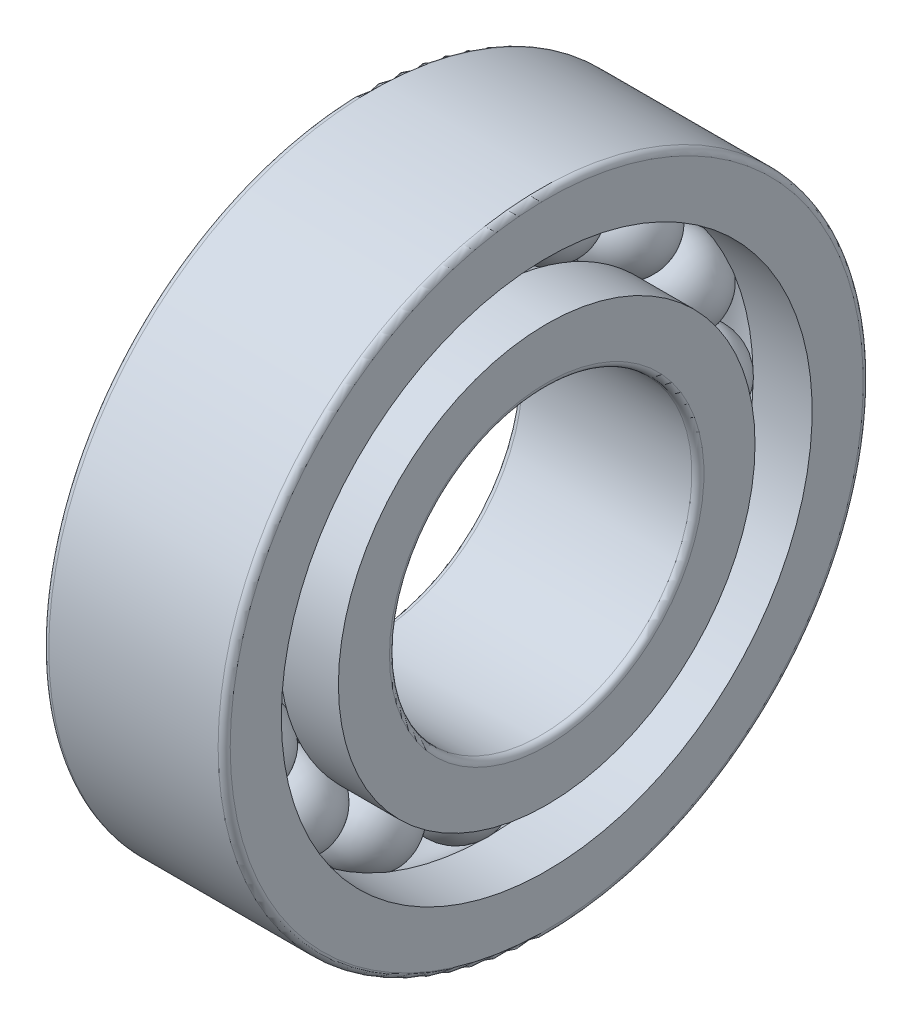
SolidWorks part; units mm, degrees
ref_plane "Front" through (0, 0, 0) normal (0, 0, 1) x (1, 0, 0)
ref_plane "Top" through (0, 0, 0) normal (0, 1, 0) x (1, 0, 0)
ref_plane "Right" through (0, 0, 0) normal (1, 0, 0) x (0, 0, -1)
sketch "Sketch1" plane through (0, 0, 0) normal (0, 0, 1) x (1, 0, 0)
  line L0 (-9.6833, 0) -> (9.8371, 0) construction
  line L1 (-2.125, 11.75) -> (2.125, 11.75)
  line L2 (-4.5966, 11.75) -> (4.6657, 11.75) construction
  arc A0 (2.125, 11.75) -> (-2.125, 11.75) centre (0, 11.75) ccw
revolve "Revolve1" add sketch "Sketch1" angle 360 about L2
sketch "Sketch2" plane through (0, 0, 0) normal (0, 0, 1) x (1, 0, 0)
  line L0 (-4.5, 10.3333) -> (-4.5, 7.5)
  line L1 (-4.5, 7.5) -> (4.5, 7.5)
  line L2 (4.5, 7.5) -> (4.5, 10.3333)
  line L3 (4.5, 10.3333) -> (1.5704, 10.3333)
  line L4 (-6.9714, 0) -> (8.1665, 0) construction
  line L5 (-6.7058, 11.75) -> (6.7058, 11.75) construction
  line L6 (-1.5704, 10.3333) -> (-4.5, 10.3333)
  arc A0 (-1.5704, 10.3333) -> (1.5704, 10.3333) centre (0, 11.75) ccw
revolve "Revolve2" add sketch "Sketch2" angle 360 about L4
sketch "Sketch3" plane through (0, 0, 0) normal (0, 0, 1) x (1, 0, 0)
  line L0 (-8.7107, 0) -> (9.1288, 0) construction
  line L1 (-4.5, 16) -> (4.5, 16)
  line L2 (-4.5, 16) -> (-4.5, 13.1667)
  line L3 (-4.5, 13.1667) -> (-1.5704, 13.1667)
  line L4 (4.5, 16) -> (4.5, 13.1667)
  line L5 (-7.2948, 11.75) -> (7.2948, 11.75) construction
  line L6 (1.5704, 13.1667) -> (4.5, 13.1667)
  arc A0 (1.5704, 13.1667) -> (-1.5704, 13.1667) centre (0, 11.75) ccw
revolve "Revolve3" add sketch "Sketch3" angle 360 about L0
pattern_circular "Circular-Pattern1" count 16 over 360 about axis through (0, 0, 0) along (1, 0, 0) of "Revolve1"
fillet "Fillet1" radius 0.3 4 edges at (-4.5, 0, 7.5) (-4.5, 0, 16) (4.5, 0, 16) (4.5, 0, 7.5)
equation "\"d0@Sketch1\" = ( \"DD@Sketch3\" + \"d@Sketch2\" )  / 2"
equation "\"dia@Sketch1\" =  ( \"DD@Sketch3\" - \"d@Sketch2\" )  / 4"
equation "\"D3@Sketch2\" = ( \"DD@Sketch3\" + \"d@Sketch2\" )  / 2 / 2"
equation "\"D4@Sketch2\" = ( \"DD@Sketch3\" - \"d@Sketch2\" )  / 6"
equation "\"D5@Sketch2\" = \"dia@Sketch1\" - 0.02"
equation "\"B/2@Sketch2\" = \"B@Sketch2\" / 2"
equation "\"D4@Sketch3\" = ( \"DD@Sketch3\" + \"d@Sketch2\" )  / 2 / 2"
equation "\"D5@Sketch3\" = ( \"DD@Sketch3\" - \"d@Sketch2\" )  / 6"
equation "\"B@Sketch3\" = \"B@Sketch2\""
equation "\"B/2@Sketch3\" = \"B@Sketch3\" / 2"
equation "\"D1@Sketch3\" = \"dia@Sketch1\" - 0.02"
equation "\"m@Circular-Pattern1\" = int( 3.14159265 / atn(( \"dia@Sketch1\" / 2) / sqr(( \"DD@Sketch3\" + \"d@Sketch2\" )  / 2 * ( \"DD@Sketch3\" + \"d@Sketch2\" )  / 2/4 - ( \"dia@Sketch1\" / 2) *  ( \"dia@Sketch1\" / 2))))-1"
